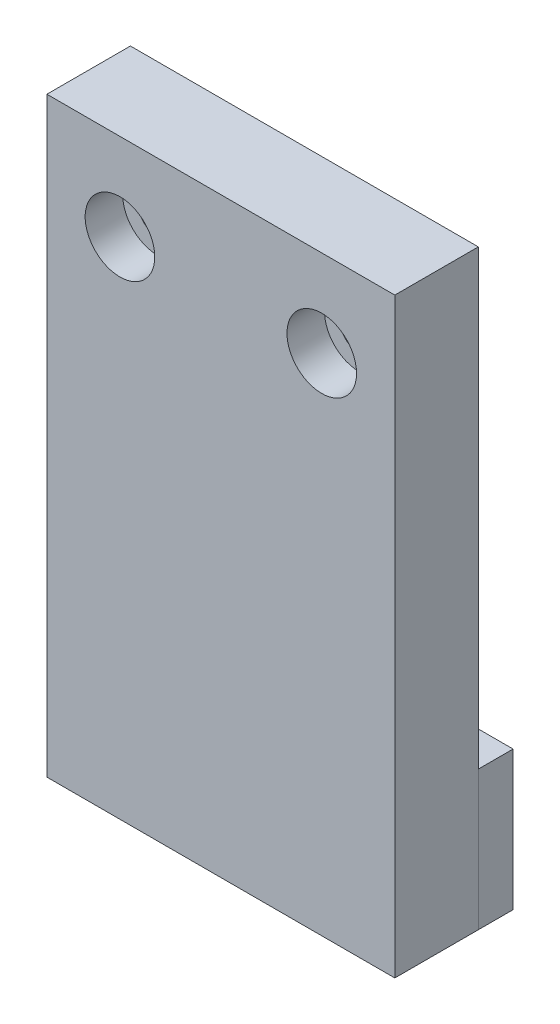
SolidWorks part; units mm, degrees
ref_plane "前视基准面" through (0, 0, 0) normal (0, 0, 1) x (1, 0, 0)
ref_plane "上视基准面" through (0, 0, 0) normal (0, 1, 0) x (1, 0, 0)
ref_plane "右视基准面" through (0, 0, 0) normal (1, 0, 0) x (0, 0, -1)
sketch "草图1" plane through (0, 0, 0) normal (0, 0, 1) x (1, 0, 0)
  line L1 (-25, -42.5) -> (25, -42.5)
  line L2 (-25, -42.5) -> (-25, 42.5)
  line L3 (-25, 42.5) -> (25, 42.5)
  line L4 (25, -42.5) -> (25, 42.5)
  line L5 (-25, -42.5) -> (25, 42.5) construction
  line L6 (-25, 42.5) -> (25, -42.5) construction
  point P0 (0, 0)
  dimension "D1" = 50
  dimension "D2" = 85
extrude "凸台-拉伸1" add sketch "草图1" along normal mid plane 12
sketch "草图2" plane through (0, 0, -6) normal (0, 0, -1) x (-1, 0, 0)
  line L0 (25, 42.5) -> (25, -42.5) construction
  line L1 (-25, -42.5) -> (25, -42.5)
  line L2 (-25, -42.5) -> (-25, -22.5)
  line L3 (-25, -22.5) -> (25, -22.5)
  line L4 (25, -42.5) -> (25, -22.5)
  dimension "D1" = 20
extrude "凸台-拉伸2" add sketch "草图2" along normal blind 5 separate body
hole_wizard "打孔尺寸(%根据)内六角圆柱头螺钉的类型1" positions "草图4" profile "草图3" counterbore size "M5" standard "GB"
sketch "草图4" plane through (0, 0, 6) normal (0, 0, 1) x (1, 0, 0)
  circle A0 centre (-14.5, 30) radius 2.067 construction
  circle A1 centre (14.5, 30) radius 2.067 construction
  point P1 (-14.5, 30)
  point P4 (14.5, 30)
sketch "草图3" plane through (-14.5, 30, 6) normal (1, 0, 0) x (0, -1, 0)
  line L0 (0, 0) -> (0, 17)
  line L1 (0, 17) -> (2.75, 17)
  line L3 (2.75, 17) -> (2.75, 5.4)
  line L4 (2.75, 5.4) -> (5, 5.4)
  line L5 (5, 5.4) -> (5, 0)
  line L7 (5, 0) -> (0, 0)
  line L11 (0, -6.35) -> (0, 107.95) construction
  dimension "通孔孔直径" = 5.5
  dimension "通孔孔深度" = 17
  dimension "柱形沉头孔直径" = 10
  dimension "柱形沉头孔深度" = 5.4
